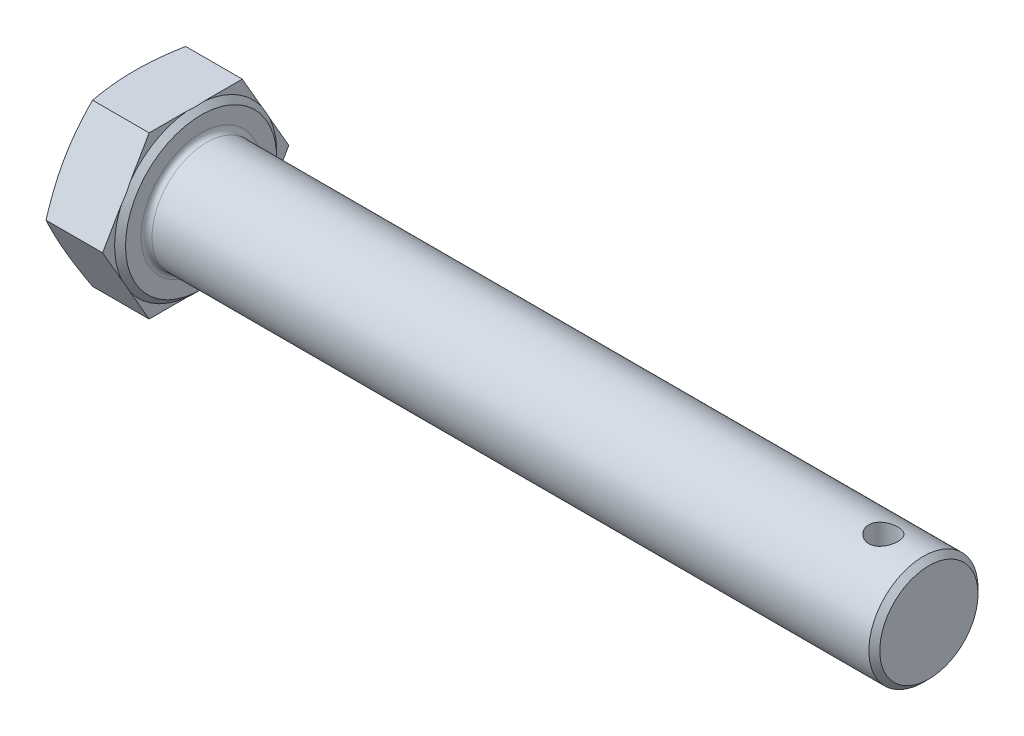
SolidWorks part; units mm, degrees
ref_plane "Front" through (0, 0, 0) normal (0, 0, 1) x (1, 0, 0)
ref_plane "Top" through (0, 0, 0) normal (0, 1, 0) x (1, 0, 0)
ref_plane "Right" through (0, 0, 0) normal (1, 0, 0) x (0, 0, -1)
other "Configuration Table"
sketch "Sketch2" plane through (0, 0, 0) normal (1, 0, 0) x (0, 0, -1)
  line L1 (10.2364, 0) -> (5.1182, 8.865)
  line L2 (5.1182, 8.865) -> (-5.1182, 8.865)
  line L3 (-5.1182, 8.865) -> (-10.2364, 0)
  line L4 (-10.2364, 0) -> (-5.1182, -8.865)
  line L5 (-5.1182, -8.865) -> (5.1182, -8.865)
  line L6 (5.1182, -8.865) -> (10.2364, 0)
  circle A0 centre (0, 0) radius 8.865 construction
extrude "BaseHead" add sketch "Sketch2" along normal blind 7.32
sketch "Sketch3" plane through (0, 0, 0) normal (0, 1, 0) x (1, 0, 0)
  line L0 (7.32, 10.2364) -> (7.32, 8.315)
  line L2 (7.32, 8.315) -> (6.72, 8.915)
  line L3 (6.72, 8.915) -> (6.72, 10.2364)
  line L5 (6.72, 10.2364) -> (7.32, 10.2364)
  line L6 (-0.9571, 0) -> (7.6478, 0) construction
  line L9 (7.32, 10.2364) -> (0, 10.2364) construction
  dimension "D1" = 45
  dimension "c" = 0.6
  dimension "dw" = 16.63
revolve "BearingFace" cut sketch "Sketch3" angle 360 about L6
sketch "Sketch4" plane through (0, 0, 0) normal (0, 1, 0) x (1, 0, 0)
  line L0 (-0.4935, 0) -> (3.5626, 0) construction
  line L2 (0, 10.2364) -> (0.4992, 10.2364)
  line L4 (0.4992, 10.2364) -> (0, 8.865)
  line L6 (0, 8.865) -> (0, 10.2364)
  line L7 (6.72, 10.2364) -> (0, 10.2364) construction
revolve "HeadChamfer" cut sketch "Sketch4" angle 360 about L0
sketch "Sketch5" plane through (7.32, 0, 0) normal (1, 0, 0) x (0, 0, -1)
  circle A0 centre (0, 0) radius 6
extrude "BaseBody" add sketch "Sketch5" along normal blind 80
cosmetic thread "ThreadCosmetic1" parameters "b"=30, "D2"=10.376
chamfer "Chamfer1" distance 0.6 angle 45 1 edges at (87.32, 0, -6)
ref_plane "Plane1" through (57.32, 0, 0) normal (1, 0, 0) x (0, 0, -1)
sketch "Sketch6" plane through (0, 0, 0) normal (0, 1, 0) x (1, 0, 0)
  line L3 (7.32, -8.315) -> (7.32, 8.315) construction
  line L4 (86.72, 0) -> (7.32, 0) construction
  circle A0 centre (82.32, 0) radius 1.6
  dimension "d1" = 3.2
  dimension "lh" = 75
extrude "Hole" cut sketch "Sketch6" against normal through all and the other way through all
fillet "HeadFillet" radius 0.6 1 edges at (7.32, 0, -6)
sketch "Sketch7" plane through (0, 0, 0) normal (0, 0, 1) x (1, 0, 0)
  line L0 (85.908, 6.2) -> (86.72, 6.2)
  line L1 (86.72, 6.2) -> (86.72, 6)
  line L2 (86.72, 6) -> (86.314, 5.2968)
  line L3 (85.908, 6) -> (86.314, 5.2968)
  line L4 (85.908, 6.2) -> (85.908, 6)
  line L5 (6.5265, 0) -> (0, 0) construction
  line L6 (85.908, 6) -> (86.72, 6) construction
  line L7 (86.314, 6) -> (86.314, 5.2968) construction
  point P5 (86.314, 6.2)
revolve "Cut-Revolve10" [suppressed] cut sketch "Sketch7" angle 360 about L5
pattern_linear "LPattern10" [suppressed] count 31 spacing 0.9744
equation "\"D2@Sketch4\" = \"s@Sketch2\""
equation "\"b@ThreadCosmetic1\" = \"l@BaseBody\" - \"lg@Plane1\""
equation "\"D1@Chamfer1\" = 0.05 * \"d@Sketch5\""
equation "\"D2@Sketch7\" = (  \"d@Sketch5\" -\"D2@ThreadCosmetic1\" )  / 2"
equation "\"D3@LPattern10\" = \"D2@Sketch7\" * 1.2"
equation "\"D1@LPattern10\" = \"b@ThreadCosmetic1\" / \"D3@LPattern10\""
